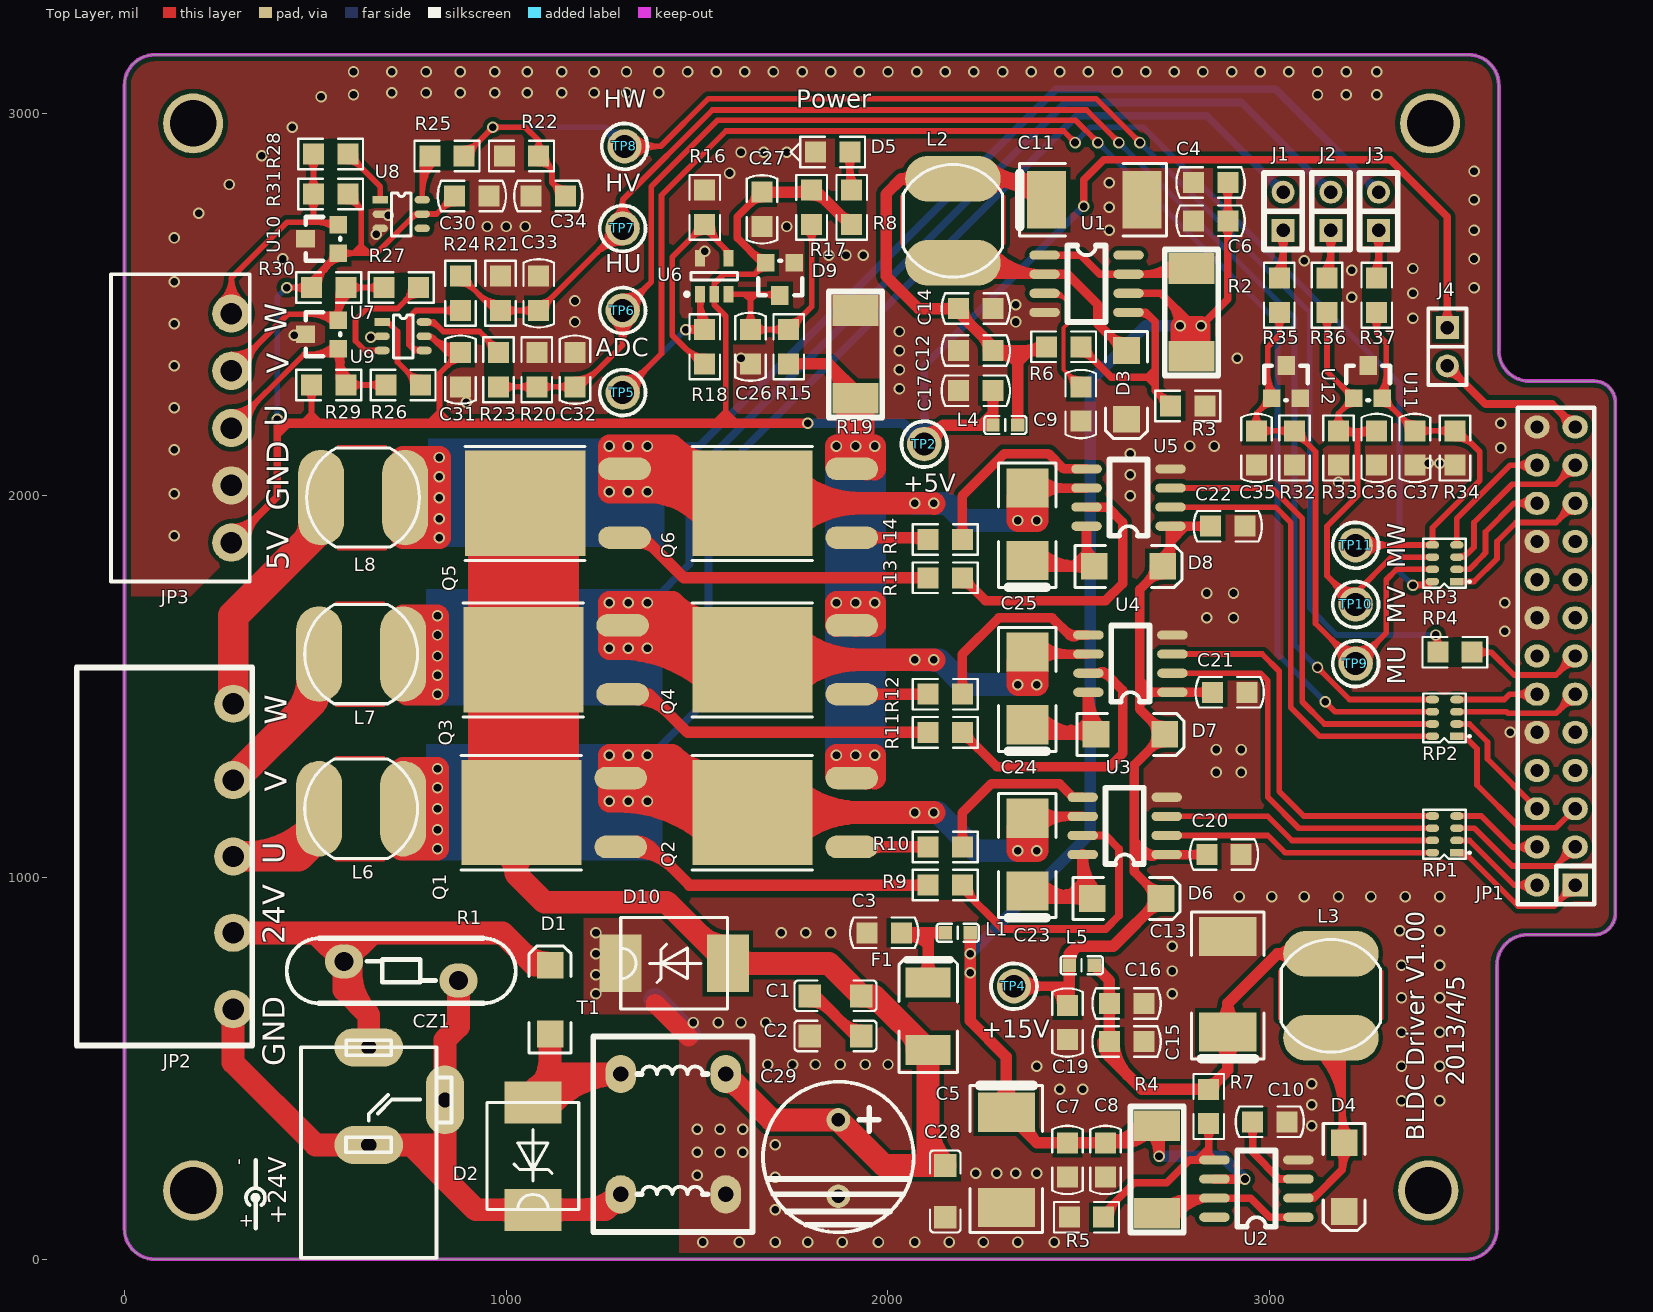
[diagram p0: Top Layer view]
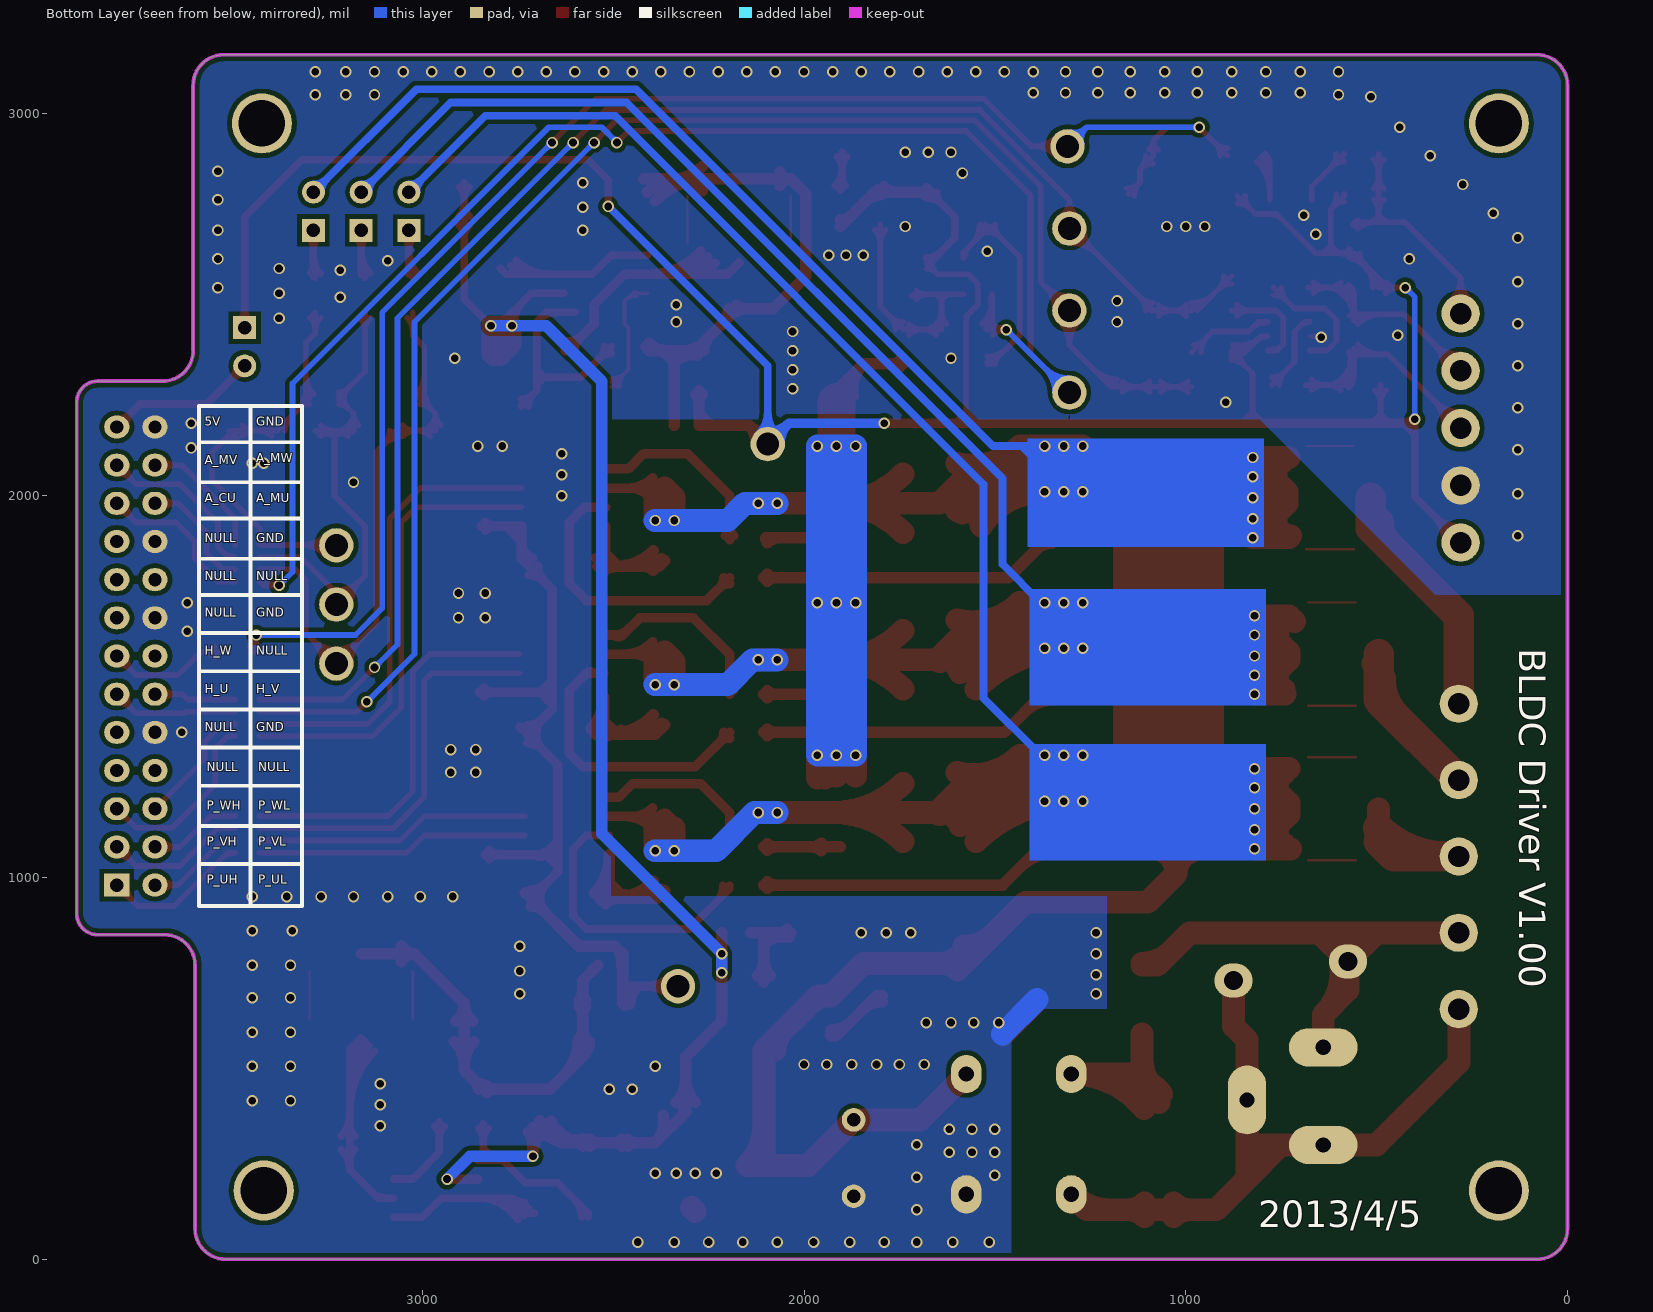
[diagram p1: Bottom Layer view, seen from below]
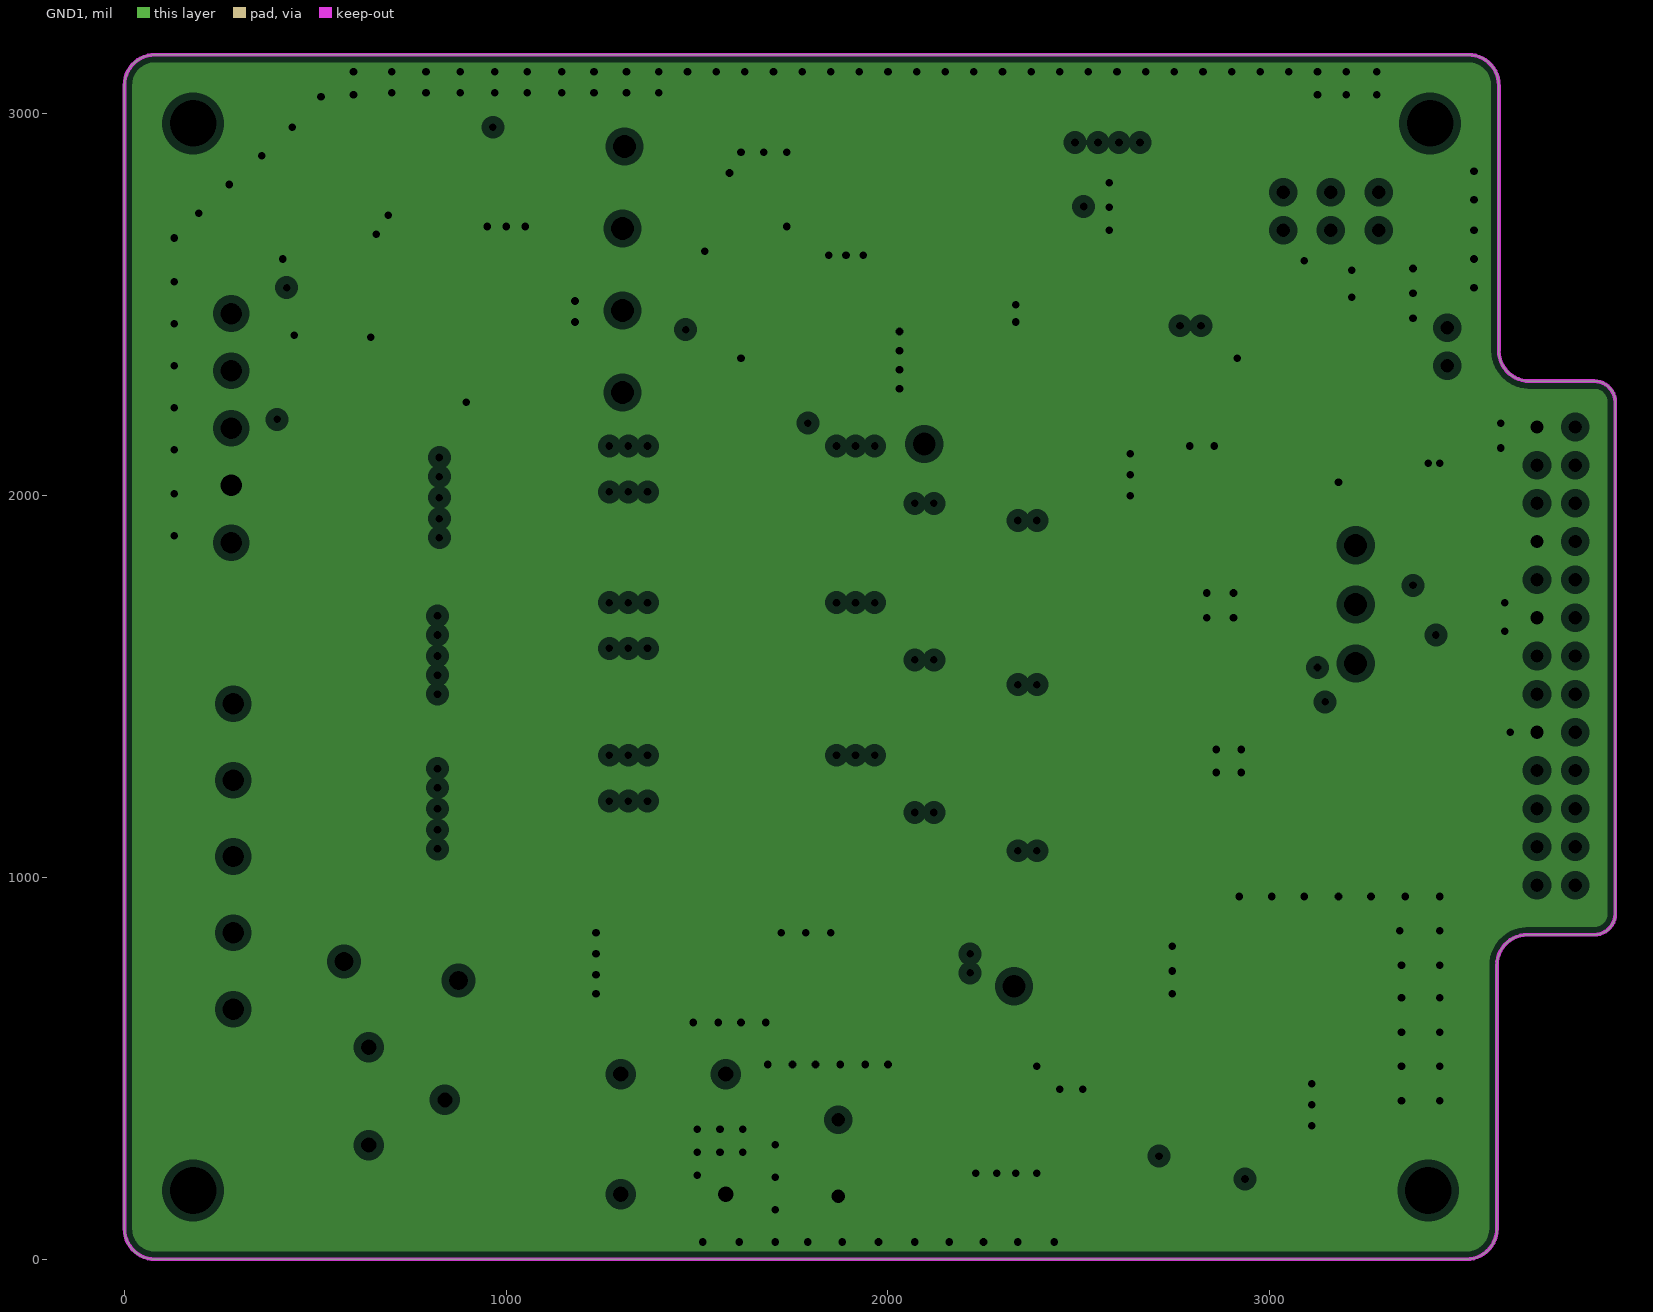
[diagram p2: GND1, clearances drawn from the general rule]
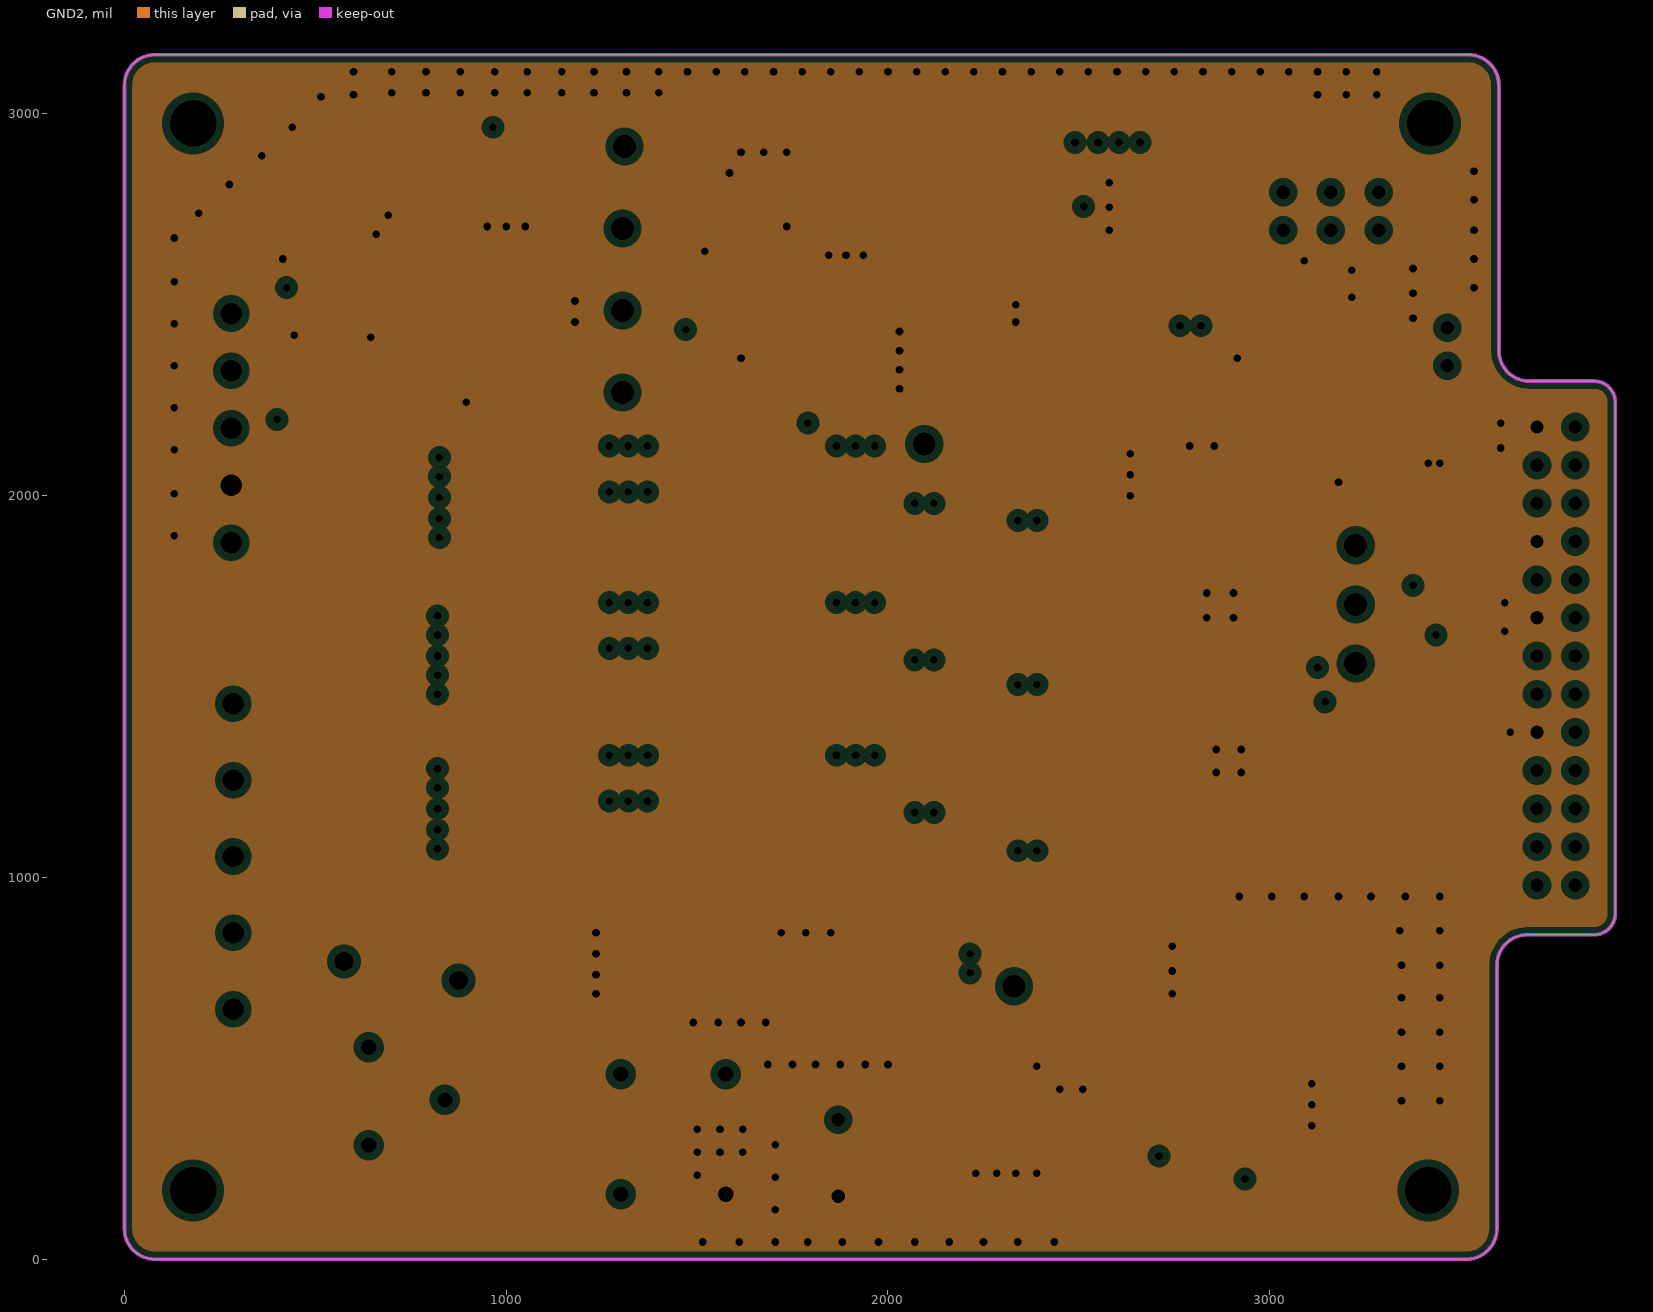
[diagram p3: GND2, clearances drawn from the general rule]
# Altium PCB MISC103926.PcbDoc (part 1 of 4)
Units mil, origin at the board's own origin, x right, y up, seen from the top; angles counter-clockwise.
Board outline 3905 x 3155 mil, 4 copper layers (Top Layer, GND1, GND2, Bottom Layer); 132 components, 84 nets, 362 pads, 268 vias.

## Layer stack, top to bottom (the 12.6 mil dielectric is the usual default, probably not edited)
Top Solder: solder mask 0.4, Solder Resist, Dk 3.5
Top Layer: signal copper 1.4
Dielectric1: core 12.6, FR-4, Dk 4.8
GND1: plane copper 1.4
Dielectric2: prepreg 12.6, FR-4, Dk 4.8
GND2: plane copper 1.4
Dielectric3: core 12.6, FR-4, Dk 4.8
Bottom Layer: signal copper 1.4
Bottom Solder: solder mask 0.4, Solder Resist, Dk 3.5

## Board outline
80,0 cw(c80,80) 0,80 0,3075 cw(c80,3075) 80,3155 3520,3155 cw(c3520,3075) 3600,3075 3600,2380 ccw(c3680,2380) 3680,2300 3850,2300 cw(c3850,2245) 3905,2245 3905,905 cw(c3850,905) 3850,850 3675,850 ccw(c3675,770) 3595,770 3595,80 cw(c3515,80) 3515,0

## Design rules (kind name [scope] priority, off if disabled: settings)
Clearance [All] p1: gap=12 ignorepadtopadclearanceinfootprint=FALSE
HoleSize [All] p1: absolutevalues=TRUE maxlimit=260 minlimit=1 maxpercent=80.000 minpercent=20.000
HoleToHoleClearance [All] p1: gap=7 allowstackedmicrovias=TRUE
MinimumSolderMaskSliver [All] p1: minsoldermaskwidth=5
PlaneClearance [All] p1: clearance=20
PlaneConnect [All] p1: planeconnectstyle=Relief reliefexpansion=20 reliefentries=4 reliefconductorwidth=10 reliefairgap=10
PolygonConnect VIA [All] p1: connectstyle=Direct reliefconductorwidth=10 reliefentries=4 polygonreliefangle="90 Angle" airgapwidth=10
PolygonConnect [All] p2: connectstyle=Direct reliefconductorwidth=10 reliefentries=4 polygonreliefangle="90 Angle" airgapwidth=10
RoutingVias [All] p1: holewidth=20 width=30 viastyle="Through Hole" minholewidth=16 minwidth=20 maxholewidth=20 maxwidth=30
SilkToSilkClearance [All] p1 off: silktosilkclearance=5
SilkToSolderMaskClearance SilkscreenOverComponentPads [IsPad] p1 off: minsilkscreentomaskgap=0 clearancetoexposedcopper=TRUE
SolderMaskExpansion [All] p1: expansion=4 istentingtop=FALSE
Width GND [InNet('GND')] p1: maxlimit=60 minlimit=8 preferedwidth=10
Width +24V [InNet('+24V')] p2: maxlimit=100 minlimit=20 preferedwidth=40
Width [All] p3: maxlimit=200 minlimit=10 preferedwidth=15
23 further rules are at their usual default settings.

## Classes and differential pairs
component class "01. ×ÜÍ¼": CZ1 J4 JP1 JP2 JP3 RP1 RP2 RP3 RP4
component class U_02: C1 C2 C3 C4 C5 C6 C7 C8 C9 C10 C11 C12 C13 C14 C15 C16 C17 C19 D1 D2 D3 D4 D5 F1 L1 L2 L3 L4 L5 R1 R2 R3 R4 R5 R6 R7 R8 T1 TP2 TP4 U1 U2
component class U_03: C20 C21 C22 C23 C24 C25 C26 C27 C28 C29 D6 D7 D8 D9 D10 L6 L7 L8 Q1 Q2 Q3 Q4 Q5 Q6 R9 R10 R11 R12 R13 R14 R15 R16 R17 R18 R19 TP5 U3 U4 U5 U6
component class U_04: C30 C31 C32 C33 C34 R20 R21 R22 R23 R24 R25 R26 R27 R28 R29 R30 R31 TP6 TP7 TP8 U7 U8 U9 U10
component class U_05: C35 C36 C37 J1 J2 J3 R32 R33 R34 R35 R36 R37 TP9 TP10 TP11 U11 U12
component class "Components Class 1": C20 C21 C22 C23 C24 C25 D6 D7 D8 R9 R10 R11 R12 R13 R14 U3 U4 U5
component class "Components Class 2": C4 C6 C9 C11 C12 C14 C17 D3 L2 L4 R3 R6 U1

## Components (designator, comment, footprint, x,y, rotation, side; value= is the part's Value field where it differs from the comment)
C1 "1nF/2KV" 1206C 1930,690 r180 top
C2 "1nF/2KV" 1206C 1930,585 r180 top
C3 "1nF" 0805C 2035,855 r180 top
C4 "100nF" 0805C 2890,2820 r180 top
C5 "100μF,50V" CAP-D 2310,385 r0 top
C6 "1nF" 0805C 2890,2720 r180 top
C7 "100nF" 0805C 2470,305 r270 top
C8 "1nF" 0805C 2570,305 r270 top
C9 "2.2nF" 0805C 2505,2285 r270 top
C10 "2.2nF" 0805C 2955,360 r0 top
C11 "47μF,25V" CAP-D 2415,2775 r90 top
C12 "100nF" 0805C 2275,2380 r180 top
C13 "100μF,50V" CAP-D 2890,595 r180 top
C14 "1nF" 0805C 2185,2490 r0 top
C15 "100nF" 0805C 2580,570 r0 top
C16 "1nF" 0805C 2580,670 r0 top
C17 "100pF" 0805C 2275,2275 r180 top
C19 "100pF" 0805C 2470,665 r270 top
C20 "100nF" 0805C 2925,1060 r180 top
C21 "100nF" 0805C 2940,1485 r180 top
C22 "100nF" 0805C 2935,1920 r180 top
C23 "10uF,25V" CAP-C 2365,965 r180 top
C24 "10uF,25V" CAP-C 2365,1400 r180 top
C25 "10uF,25V" CAP-C 2365,1830 r180 top
C26 "10nF" 0805C 1640,2345 r90 top
C27 "100nF" 0805C 1670,2705 r90 top
C28 "1nF/2KV" 1206C 2150,245 r270 top
C29 "330μF,50V" µç½âµçÈÝ 1870,260 r90 top
C30 "100nF" 0805C 865,2785 r0 top
C31 "100nF" 0805C 880,2285 r90 top
C32 "100pF" 0805C 1180,2285 r90 top
C33 "100pF" 0805C 1085,2485 r90 top
C34 "100pF" 0805C 1155,2785 r180 top
C35 "10nF" 0805C 2965,2080 r90 top
C36 "10nF" 0805C 3280,2080 r90 top
C37 "10nF" 0805C 3380,2080 r90 top
CZ1 "POWER" POWER-AC 640,555 r270 top
D1 "SK310A" DO-214AC 1115,590 r90 top
D2 "1SMC30AT3" 1SMC17AT 1070,270 r90 top
D3 "SK310A" DO-214AC 2625,2380 r270 top
D4 "SK310A" DO-214AC 3195,305 r270 top
D5 "Power" 0805D 1900,2900 r180 top
D6 "SK310A" DO-214AC 2535,945 r0 top
D7 "SK310A" DO-214AC 2545,1375 r0 top
D8 "SK310A" DO-214AC 2540,1815 r0 top
D9 "BAT54S" SOT-23 1755,2610 r180 top
D10 "1SMC30AT3" 1SMC17AT 1440,775 r0 top
F1 "SMD050" 1812DT 2105,725 r270 top
J1 "CON2" SIP-2 3035,2695 r90 top
J2 "CON2" SIP-2 3160,2695 r90 top
J3 "CON2" SIP-2 3285,2695 r90 top
J4 "CON2" SIP-2 3465,2440 r270 top
JP1 "HDR13×2" IDC-26 3800,980 r90 top
JP2 "CON5" CON-5-5.0 285,655 r90 top
JP3 "CON5" CON-5-3.81 280,1875 r90 top
L1 "CBG160808U121T" 0603C 2150,855 r0 top
L2 "220uH" L-7.5S 2170,2610 r180 top
L3 "220uH" L-7.5S 3160,580 r180 top
L4 "CBG160808U121T" 0603C 2340,2185 r180 top
L5 "CBG160808U121T" 0603C 2540,770 r180 top
L6 "47uH" L-7.5S 730,1180 r270 top
L7 "47uH" L-7.5S 730,1585 r270 top
L8 "47uH" L-7.5S 735,1995 r270 top
Q1 "NTD32N06" DPAK-3 1300,1080 r90 top
Q2 "NTD32N06" DPAK-3 1905,1080 r90 top
Q3 "NTD32N06" DPAK-3 1305,1480 r90 top
Q4 "NTD32N06" DPAK-3 1905,1480 r90 top
Q5 "NTD32N06" DPAK-3 1310,1890 r90 top
Q6 "NTD32N06" DPAK-3 1905,1890 r90 top
R1 "330KD14" AX-.3/.6 575,780 r90 top
R2 "0.18Ω" 2512 2795,2365 r90 top
R3 "2.2KΩ" 0805R 2740,2235 r0 top
R4 "0.18Ω" 2512 2705,350 r270 top
R5 "1KΩ" 0805R 2565,110 r180 top
R6 "6.8KΩ,1%" 0805R 2505,2390 r180 top
R7 "11KΩ,1%" 0805R 2840,355 r90 top
R8 "2KΩ" 0805R 1905,2710 r90 top
R9 "33Ω" 0805R 2195,980 r180 top
R10 "33Ω" 0805R 2195,1080 r180 top
R11 "33Ω" 0805R 2195,1380 r180 top
R12 "33Ω" 0805R 2195,1480 r180 top
R13 "33Ω" 0805R 2195,1785 r180 top
R14 "33Ω" 0805R 2195,1885 r180 top
R15 "1KΩ" 0805R 1740,2435 r270 top
R16 "150KΩ" 0805R 1520,2710 r90 top
R17 "20KΩ" 0805R 1800,2800 r270 top
R18 "300KΩ" 0805R 1520,2435 r270 top
R19 "0.33Ω" 2512 1915,2485 r270 top
R20 "10KΩ" 0805R 1080,2375 r270 top
R21 "10KΩ" 0805R 985,2575 r270 top
R22 "10KΩ" 0805R 995,2890 r0 top
R23 "6.8KΩ" 0805R 980,2285 r90 top
R24 "6.8KΩ" 0805R 880,2575 r270 top
R25 "6.8KΩ" 0805R 890,2890 r180 top
R26 "33Ω" 0805R 775,2290 r180 top
R27 "33Ω" 0805R 770,2545 r180 top
R28 "33Ω" 0805R 585,2895 r180 top
R29 "4.7KΩ" 0805R 580,2290 r180 top
R30 "4.7KΩ" 0805R 580,2545 r180 top
R31 "4.7KΩ" 0805R 495,2790 r0 top
R32 "10KΩ" 0805R 3065,2170 r270 top
R33 "10KΩ" 0805R 3180,2170 r270 top
R34 "10KΩ" 0805R 3485,2170 r270 top
R35 "100KΩ" 0805R 3025,2570 r270 top
R36 "100KΩ" 0805R 3150,2570 r270 top
R37 "100KΩ" 0805R 3280,2570 r270 top
RP1 "33Ω" PZ-4-0.8B 3490,1065 r180 top
RP2 "33Ω" PZ-4-0.8B 3490,1370 r180 top
RP3 "33Ω" PZ-4-0.8B 3490,1775 r180 top
RP4 "33Ω" 0805R 3530,1590 r180 top
T1 "Com Tra" L-2-XIAO 1300,170 r180 top
TP2 "+5V" PAD(60) 2095,2135 r0 top
TP4 "+15V" PAD(60) 2330,715 r0 top
TP5 "ADC" PAD(60) 1305,2270 r0 top
TP6 "HU" PAD(60) 1305,2485 r180 top
TP7 "HV" PAD(60) 1305,2700 r180 top
TP8 "HW" PAD(60) 1310,2915 r180 top
TP9 "MU" PAD(60) 3225,1560 r180 top
TP10 "MV" PAD(60) 3225,1715 r270 top
TP11 "MW" PAD(60) 3225,1870 r180 top
U1 "NCP3063" SO-8 2410,2630 r0 top
U2 "NCP3063" SO-8 3075,110 r180 top
U3 "NCP5106B" SO-8 2730,1060 r180 top
U4 "NCP5106B" SO-8 2745,1485 r180 top
U5 "NCP5106B" SO-8 2740,1920 r180 top
U6 "LMC7101QM5" MF05A_N 1545,2575 r90 top
U7 "SN74LVC2G14DBVR" SOT-23-6 675,2455 r0 top
U8 "SN74LVC2G14DBVR" SOT-23-6 670,2775 r0 top
U9 "PESD5V2S2UT" SOT-23 560,2385 r90 top
U10 "PESD5V2S2UT" SOT-23 560,2635 r90 top
U11 "PESD3V3S2UT" SOT-23 3220,2255 r0 top
U12 "PESD3V3S2UT" SOT-23 3005,2255 r0 top

## Footprints (in the part's own frame and the unit in brackets; to place one, negate y for a bottom-side part, rotate by r counter-clockwise, add the part's x,y. Pads: shape width x height; smd on the part's side, far side on the other; paste and mask are expansions set on the pad)
1SMC17AT [mil]
  rect 110x150 smd: 1(140.5,0) 2(-140.5,0)
  silkscreen extent -140,-120 140,120
0603C [mil]
  rect 35x35 smd: 1(0,0) 2(65,0)
  silkscreen extent -23,-24 88,24
0805C [mil]
  rect 55x55 smd: 1(0,0) 2(90,0)
  silkscreen extent -44,-40 134,40
0805D [mil]
  rect 55x55 smd: 1(0,0) 2(90,0)
  silkscreen extent -40,-40 155,40
0805R [mil]
  rect 55x55 smd: 1(0,0) 2(90,0)
  silkscreen extent -40,-40 130,40
1206C [mil]
  rect 60x60 smd: 1(0,0) 2(135,0)
  silkscreen extent -40,-40 175,40
1812DT [mm]
  rect 2x3 smd: 1(4.496,0) 2(0,0)
  silkscreen extent -1.63,-1.95 5.99,1.97
2512 [mil]
  rect 80x120 smd: 1(0,0) 2(230,0)
  silkscreen extent -50,-70 280,70
AX-.3/.6 [mil]
  oval 90x100 hole 50: 1(0,0) 2(-50,-300)
  silkscreen extent -109,-450 61,150
CAP-C [mm]
  rect 2.8x2.6 smd: 1(0,0) 2(0,-4.826)
  silkscreen extent -1.91,-6.48 1.91,1.78
CAP-D [mm]
  rect 3.8x2.6 smd: 1(0,0) 2(0,-6.35)
  silkscreen extent -2.41,-8 2.41,1.78
CON-5-3.81 [mil]
  round 100 hole 56: 1(2,0) 2(152,0) 3(302,0) 4(452,0) 5(602,0)
  silkscreen extent -100,-48 705,315
CON-5-5.0 [mil]
  round 100 hole 56: 1(0,0) 2(200,0) 3(400,0) 4(600,0) 5(800,0)
  silkscreen extent -95,-50 895,410
DO-214AC [mil]
  rect 70x70 smd: 1(0,0) 2(180,0)
  silkscreen extent -50,-55 230,55
DPAK-3 [mm]
  oval 1.5x3.5 smd: 1(0,0) 3(4.58,0)
  rect 7x8 smd: 2(2.29,6.604)
  silkscreen extent -1.52,2.62 6.07,10.62
IDC-26 [mil]
  rect 60x66 hole 35: 1(0,0)
  oval 60x66 hole 35: 2(0,100) 3(100,0) 4(100,100) 5(200,0) 6(200,100) 7(300,0) 8(300,100) 9(400,0) 10(400,100) 11(500,0) 12(500,100) 13(600,0) 14(600,100) 15(700,0) 16(700,100) 17(800,0) 18(800,100) 19(900,0) 20(900,100) 21(1000,0) 22(1000,100) 23(1100,0) 24(1100,100) 25(1200,0) 26(1200,100)
  silkscreen extent -50,-50 1250,150
L-2-XIAO [mil]
  oval 80x100 hole 40: 1(0,0) 2(-275,0) 3(-275,-315) 4(0,-315)
  silkscreen extent -345,-413 72,98
L-7.5S [mil]
  oval 250x120 smd: 1(0,0) 2(0,-220)
  Top Layer lines w6: 135,-50 135,-175 ; -135,-50 -135,-175
  silkscreen extent -130,-258 130,38
MF05A_N [mm] "SOT23, 5-Leads, Body 2.9x1.6mm, Pitch 0.95mm, Lead Span 2.8mm, IPC Med"
  rect 1.1x0.65 smd: 1(-1.2,0.95) 2(-1.2,0) 3(-1.2,-0.95) 4(1.2,-0.95) 5(1.2,0.95)
  silkscreen extent -1.32,-1.55 0.25,1.95, body extent -0.9,-1.55 0.9,1.55, height 1.22
PAD(60) [mil]
  round 90 hole 60: 1(0,0)
  silkscreen extent -60,-60 60,60
POWER-AC [mil]
  oval 180x100 hole 40: 1(137.8,199.37)
  oval 100x180 hole 40: 2(0,0) 3(255.91,0)
  silkscreen extent -18,-177 551,217
PZ-4-0.8B [mil]
  rect 35x20 smd: 1(0,0)
  oval 35x20 smd: 2(0,-32) 3(0,-64) 4(0,-96) 5(64,-96) 6(64,-64) 7(64,-32) 8(64,0)
  silkscreen extent -34,-112 88,16
SIP-2 [mil]
  rect 60x60 hole 35: 1(0,0)
  round 60 hole 35: 2(100,0)
  silkscreen extent -50,-50 150,50
SO-8 [mil]
  oval 80x24 smd: 1(0,0) 2(0,-50) 3(0,-100) 4(0,-150) 5(220,-150) 6(220,-100) 7(220,-50) 8(220,0)
  silkscreen extent 60,-175 160,25
SOT-23 [mil]
  rect 46x46 smd: 1(0,0) 2(75,0)
  rect 46x50 smd: 3(38,86)
  silkscreen extent -20,-5 95,85
SOT-23-6 [mil]
  rect 40x20 smd: 1(0,0)
  oval 40x20 smd: 2(0,-37.4) 3(0,-74.8) 4(110,-74.8) 5(110,-37.4) 6(110,0)
  silkscreen extent 30,-94 81,18
µç½âµçÈÝ [mil]
  round 62 hole 35: 1(105,0) 2(-95,0)
  silkscreen extent -190,-197 205,197

## Part data
F1: library part Fuse
JP2: library part M
JP3: library part MHDR1X5, "He"
L1 L2 L3 L4 L5 L6 L7 L8: library part Induct
U6: "Tiny Low Power Operational Amplifier with Rail-to-Rail Input and Output"

## Free pads (board coordinates)
  round 157.48 hole 122.05: 0(180,180) 0(180,2975) 0(3415,180) 0(3420,2975)

## Via types
v1: diameter 30, hole 20, Top Layer to Bottom Layer, 268 vias

## Nets (pads, with @x,y where several pads share a name; then routed paths per layer and width w, separated by ;. In a path a pad name is that pad's centre, name@x,y a point inside that pad or via, vN(x,y) a via of type N, cw(c..) or ccw(c..) an arc to the next point about the centre after c; other vN are vias at no path point)
+5V: C17.1 C27.2 C30.1 C31.2 D9.2 J4.1 JP3.1 L4.2 R8.1 R17.1 R29.2 R30.2 R31.2 TP2.1 U6.2 U7.5 U8.5 U10.1 | length 9532.1
  Top Layer w15: v1(400,2200) v1@410,2190 ; v1(425,2545) R30.2@490,2545 490,2565 U10.1@560,2635 660,2635 762.6,2737.6 U8.5@780,2737.6 817.6,2737.6 C30.1@865,2785 ; v1@430.3,2539.7 cw(c443.11,2526.89) 443.11,2545 cw(c443.11,2563.11) v1@430.3,2550.3 ; 465,2190 490,2215 ; R29.2@475.86,2275.86 cw(c441.72,2241.72) 490,2241.72 cw(c538.28,2241.72) R29.2@504.14,2275.86 ; R30.2@475.86,2530.86 ccw(c441.72,2496.72) 441.72,2545 ccw(c441.72,2593.28) R30.2@475.86,2559.14 ; 490,2190 490,2215 ; R29.2@490,2290 490,2215 ; R30.2@495,2545 cw(c555.35,2545) 512.68,2587.68 ; 510,2190 510,2195 490,2215 ; R30.2@510,2545 cw(c606.57,2545) U10.1@538.28,2613.28 ; 525.11,2591.34 cw(c578.98,2559.01) U10.1@563.76,2619.96 ; U10.1@544.5,2635 cw(c507.08,2635) 533.54,2608.54 cw(c560,2582.08) U10.1@560,2619.5 ; U10.1@570.96,2624.04 cw(c597.42,2597.58) 597.42,2635 cw(c597.42,2672.42) U10.1@570.96,2645.96 ; R31.2@585,2770 cw(c585,2733.79) 610.61,2759.39 ; R31.2@585,2790 585,2785 620,2750 ; 600,2635 620,2655 ; R31.2@604.97,2789 ccw(c656.42,2786.43) 620,2750 ; 620,2635 620,2655 ; 640,2635 620,2655 ; 753.1,2728.1 cw(c770,2711.19) U8.5@770,2735.1 ; U7.5@785,2417.6 U7.5@802.4,2417.6 ; U7.5@795,2415.1 cw(c795,2391.19) 811.9,2408.1 ; U7.5@795.65,2415.18 cw(c800.48,2397.15) 809.81,2413.32 ; 800,2190 800,2195 825,2220 ; 822.55,2397.45 ccw(c867.47,2442.37) C31.2@879.09,2379.92 ; 825,2190 825,2220 ; 842.69,2377.31 ccw(c873.79,2408.4) C31.2@881.83,2365.17 ; C30.1@845,2785 cw(c796.72,2785) 830.86,2750.86 cw(c865,2716.72) C30.1@865,2765 ; 850,2190 850,2195 825,2220 ; C31.2@860,2375 cw(c811.72,2375) 845.86,2340.86 cw(c880,2306.72) C31.2@880,2355 ; C31.2@862.77,2364.85 ccw(c845,2354.38) 845,2375 ; C31.2@862.77,2385.15 cw(c845,2395.62) 845,2375 ; C31.2@876.34,2394.66 cw(c861.15,2476.34) U7.5@802.41,2417.59 ; 1545,2190 1575,2220 ; 1575,2190 1575,2220 ; 1605,2190 1575,2220 ; D9.2@1664.5,2610 cw(c1627.08,2610) 1653.54,2583.54 cw(c1680,2557.08) D9.2@1680,2594.5 ; D9.2@1670,2610 D9.2@1680,2610 1650,2580 1570,2580 1545,2555 U6.2@1545,2527.76 1545,2500 1575,2470 1575,2220 ; R17.1@1795,2795 R17.1@1800,2800 R17.1@1810,2800 ; 620,2655 620,2750 ; U7.5@802.4,2417.6 845,2375 ; 825,2220 825,2320 C31.2@880,2375 845,2375
  Top Layer w20: JP3.1@280,1877 400,1997 v1(400,2200) ; JP3.1@280,1917 ccw(c280,2013.57) 348.28,1945.28 ccw(c416.57,1877) JP3.1@320,1877 ; 400,2160 430,2190 ; 1640.74,2639.26 ccw(c1680,2678.53) D9.2@1680,2623 ; C27.2@1652.5,2795 cw(c1610.25,2795) 1640.13,2765.13 cw(c1670,2735.25) C27.2@1670,2777.5 ; D9.2@1670,2610 1605,2675 1605,2730 C27.2@1670,2795 ; v1(2512.5,2757.5) 2512.5,2827.5 2565,2880 3315,2880 3465,2730 J4.1@3465,2440 ; J4.1@3450.86,2454.14 ccw(c3416.71,2488.28) 3465,2488.28 ccw(c3513.28,2488.28) J4.1@3479.14,2454.14
  Top Layer w25: v1@401.78,2201.76 ccw(c430,2229.75) 430,2190 ; v1@410,2190 430,2190 ; v1(1790,2190) 1605,2190 1575,2190 1545,2190 850,2190 825,2190 800,2190 510,2190 490,2190 465,2190 430,2190
  Top Layer w30: C27.2@1670,2795 R17.1@1795,2795 ; C27.2@1678.84,2786.16 cw(c1700.18,2764.82) 1700.18,2795 cw(c1700.18,2825.18) C27.2@1678.84,2803.84 ; 1757.75,2795 ccw(c1757.75,2842.25) R17.1@1791.16,2808.84 ; R17.1@1800,2787.5 cw(c1800,2733.18) 1838.41,2771.59 ; R17.1@1810,2800 R8.1@1905,2705 ; 1875.13,2734.87 ccw(c1905,2764.75) R8.1@1905,2722.5 ; TP2.1@2095.51,2165 ccw(c2096.68,2233.31) 2145,2185 ; TP2.1@2100,2140 2145,2185 ; TP2.1@2125,2135.51 cw(c2193.31,2136.69) 2145,2185 ; C17.1@2266.16,2266.16 cw(c2244.82,2244.82) 2275,2244.82 cw(c2305.18,2244.82) C17.1@2283.84,2266.16 ; 2275,2215 2245,2185 ; C17.1@2275,2275 L4.2@2275,2185 2245,2185 ; 2145,2185 2245,2185
  Bottom Layer w15: v1@394.7,2205.3 ccw(c381.89,2218.11) 400,2218.11 ccw(c418.11,2218.11) v1@405.3,2205.3 ; v1(400,2200) 400,2520 v1(425,2545) ; v1@417.5,2545 cw(c399.39,2545) 412.2,2532.2 cw(c425,2519.39) v1@425,2537.5
  Bottom Layer w20: TP2.1@2070.25,2159.75 ccw(c2010.5,2219.5) 2095,2219.5 ccw(c2179.5,2219.5) TP2.1@2119.75,2159.75 ; TP2.1@2095,2135 2095,2340 v1(2512.5,2757.5)
  Bottom Layer w25: v1(1790,2190) 2040,2190 ; TP2.1@2062.5,2135.2 ccw(c1985.68,2135.68) 2040,2190 ; TP2.1@2094.8,2167.5 cw(c2094.32,2244.32) 2040,2190 ; TP2.1@2095,2135 2040,2190
+15V: C19.1 C20.2 C21.2 C22.2 D6.2 D7.2 D8.2 L5.2 TP4.1 U3.1 U4.1 U5.1 | length 3571.3
  Top Layer w25: TP4.1@2330,715 2430,715 ; TP4.1@2352.98,692.02 cw(c2408.46,636.54) 2408.46,715 cw(c2408.46,793.46) TP4.1@2352.98,737.98 ; 2437.32,707.68 cw(c2394.65,665) C19.1@2455,665 ; C19.1@2475,670 2430,715 ; 2475,715 2430,715 ; 2645,1030 2675,1060 2680,1060 ; 2645,1060 2680,1060 ; 2645,1090 2650,1090 2680,1060 ; 2660,1460 2665,1460 2690,1485 ; 2660,1490 2665,1485 2690,1485 ; 2660,1510 2665,1510 2690,1485 ; 2665,1060 2680,1060 ; 2665.3,1074.7 ccw(c2702,1111.41) U3.1@2702,1059.5 ; D6.2@2692.5,945 ccw(c2638.18,945) 2676.59,983.41 ccw(c2715,1021.82) D6.2@2715,967.5 ; D8.2@2697.5,1815 cw(c2643.18,1815) 2681.59,1776.59 cw(c2720,1738.18) D8.2@2720,1792.5 ; U3.1@2702.34,1059.64 cw(c2691.36,1071.36) 2680,1060 ; D8.2@2710.98,1835.61 ccw(c2691.55,1880) 2740,1880 ; D6.2@2715,945 2645,1015 2645,1295 D7.2@2725,1375 ; D7.2@2725,1352.5 ccw(c2725,1298.18) 2686.59,1336.59 ccw(c2648.18,1375) 2702.5,1375 ccw(c2648.18,1375) 2686.59,1413.41 ccw(c2725,1451.82) D7.2@2725,1397.5 ; U5.1@2740.36,1920.35 cw(c2719.65,1900.36) 2740,1880 ; D7.2@2745,1395 D7.2@2725,1375 ; U5.1@2780,1920 2740,1880 ; C20.2@2824.39,1049.39 ccw(c2798.79,1023.79) 2798.79,1060 ccw(c2798.79,1096.21) C20.2@2824.39,1070.61 ; C22.2@2834.39,1909.39 ccw(c2808.79,1883.79) 2808.79,1920 ccw(c2808.79,1956.21) C22.2@2834.39,1930.61 ; C20.2@2835,1060 U3.1@2730,1060 2680,1060 ; C21.2@2839.39,1474.39 ccw(c2813.79,1448.79) 2813.79,1485 ccw(c2813.79,1521.21) C21.2@2839.39,1495.61 ; C22.2@2845,1920 U5.1@2740,1920 2740,1880 ; C21.2@2850,1485 U4.1@2745,1485 2690,1485 ; D8.2@2720,1815 2660,1755 2660,1440 D7.2@2725,1375 ; D8.2@2720,1815 D8.2@2740,1835 ; D8.2@2720,1815 D8.2@2740,1835 ; D8.2@2740,1835 2740,1880
  Top Layer w30: C19.1@2461.16,673.84 ccw(c2427.75,707.25) 2475,707.25 ; C19.1@2470,665 2475,670 L5.2@2475,770 2475,800 2495,820 ; L5.2@2477.49,770.27 cw(c2538.14,776.86) 2495,820 ; D6.2@2695,945 cw(c2646.72,945) 2680.86,910.86 cw(c2715,876.72) D6.2@2715,925 ; D6.2@2730,960 D6.2@2715,945 2590,820 2495,820
+24V: C1.1 C28.1 C29.1 D10.1 F1.1 Q1.2 Q3.2 Q5.2 T1.3 | length 3088.6
  Top Layer w60: Q1.2@983.69,1068.77 cw(c962.44,1009.94) 1025,1009.94 cw(c1093.24,1009.94) Q1.2@1064.97,1072.05 ; Q1.2@1015,1185.16 1025,1175.16 1025,1010 1100,935 1420.5,935 D10.1@1580.5,775 1845,775 C1.1@1930,690 ; 1503.68,851.82 ccw(c1580.5,928.64) D10.1@1580.5,820 ; T1.3@1575,465 cw(c1575,416.72) 1609.14,450.86 ; T1.3@1575,485 1695,365 C29.1@1870,365 1990,245 C28.1@2150,245 cw(c2258.64,353.64) 2105,353.64 ; D10.1@1598.18,757.32 cw(c1640.86,714.64) 1640.86,775 cw(c1640.86,835.36) D10.1@1598.18,792.68 ; 1986.34,666.66 ccw(c1930,610.33) C1.1@1930,690 ; 2055.4,597.6 cw(c2005.8,548) F1.1@2075.95,548 ; 2105,245 F1.1@2105,548 1963,690 C1.1@1930,690
  Top Layer w100: Q1.2@1015,1185.16 Q1.2@1050,1220.16